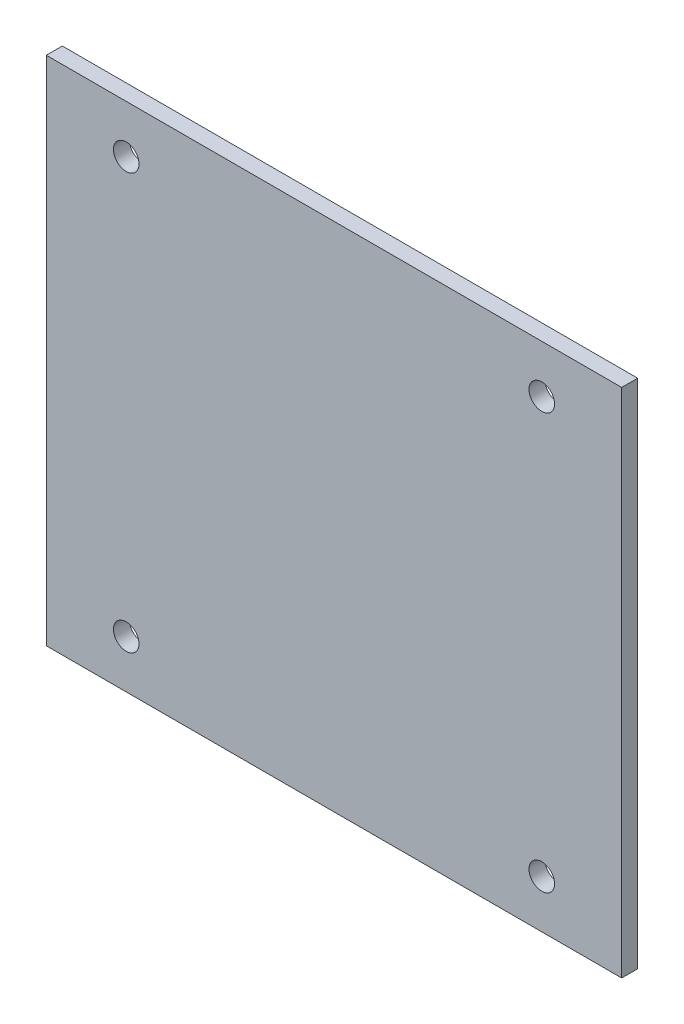
from build123d import *

# Parameters (mm, degrees)
SKETCH_1_W          = 180
SKETCH_1_H          = 160
EXTRUDE_1_DEPTH     = 5
SKETCH_2_R          = 4
CUT_EXTRUDE_1_DEPTH = 121.519707932


with BuildPart() as part:
    # 草图1 → 凸台-拉伸1 (new body)
    with BuildSketch(Plane.XY):
        Rectangle(SKETCH_1_W, SKETCH_1_H)
    extrude(amount=EXTRUDE_1_DEPTH)

    # 草图2 → 切除-拉伸1 (cut, through all)
    with BuildSketch(Plane.XY.offset(5)):
        with Locations((-65, 65)):
            Circle(SKETCH_2_R)
        with Locations((65, 65)):
            Circle(SKETCH_2_R)
        with Locations((65, -65)):
            Circle(SKETCH_2_R)
        with Locations((-65, -65)):
            Circle(SKETCH_2_R)
    extrude(amount=-CUT_EXTRUDE_1_DEPTH, mode=Mode.SUBTRACT)


solid = part.part
